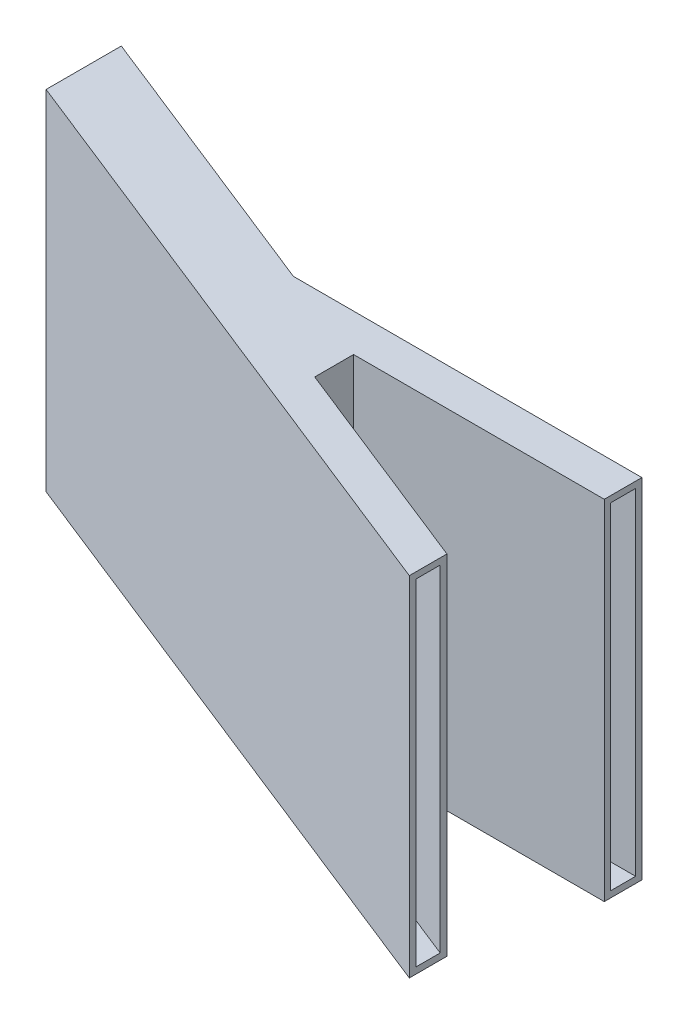
from build123d import *

# Parameters (mm, degrees)
BOSS_EXTRUDE1_DEPTH = 556
SHELL1_T            = -10
SKETCH2_W           = 100
SKETCH2_H           = 444.236647894
CUT_EXTRUDE1_DEPTH  = 15


with BuildPart() as part:
    # Sketch1 → Boss-Extrude1 (new body)
    with BuildSketch(Plane(origin=(0, 0, 0), x_dir=(1, 0, 0), z_dir=(0, 1, 0))):
        Polygon((100, 0), (500, 0), (500, 60), (-56, 60), (-511.593220339, 241.016949153), (-511.593220339, 121.016949153), (450, -261.044642857), (450, -201.044642857), (100, -61.982142857), align=None)
    extrude(amount=BOSS_EXTRUDE1_DEPTH)

    # Shell1
    shell1_openings = [part.faces().sort_by_distance(p)[0] for p in [
        (450, 278, 231.044642857),
        (-511.593220339, 278, -181.016949153),
        (500, 278, -30),
    ]]
    offset(amount=SHELL1_T, openings=shell1_openings, kind=Kind.INTERSECTION)

    # Sketch2 → Cut-Extrude1 (cut)
    with BuildSketch(Plane(origin=(0, 0, -60), x_dir=(-1, 0, 0), z_dir=(0, 0, -1))):
        with Locations((6, 263.213951143)):
            Rectangle(SKETCH2_W, SKETCH2_H)
    extrude(amount=-CUT_EXTRUDE1_DEPTH, mode=Mode.SUBTRACT)


solid = part.part
